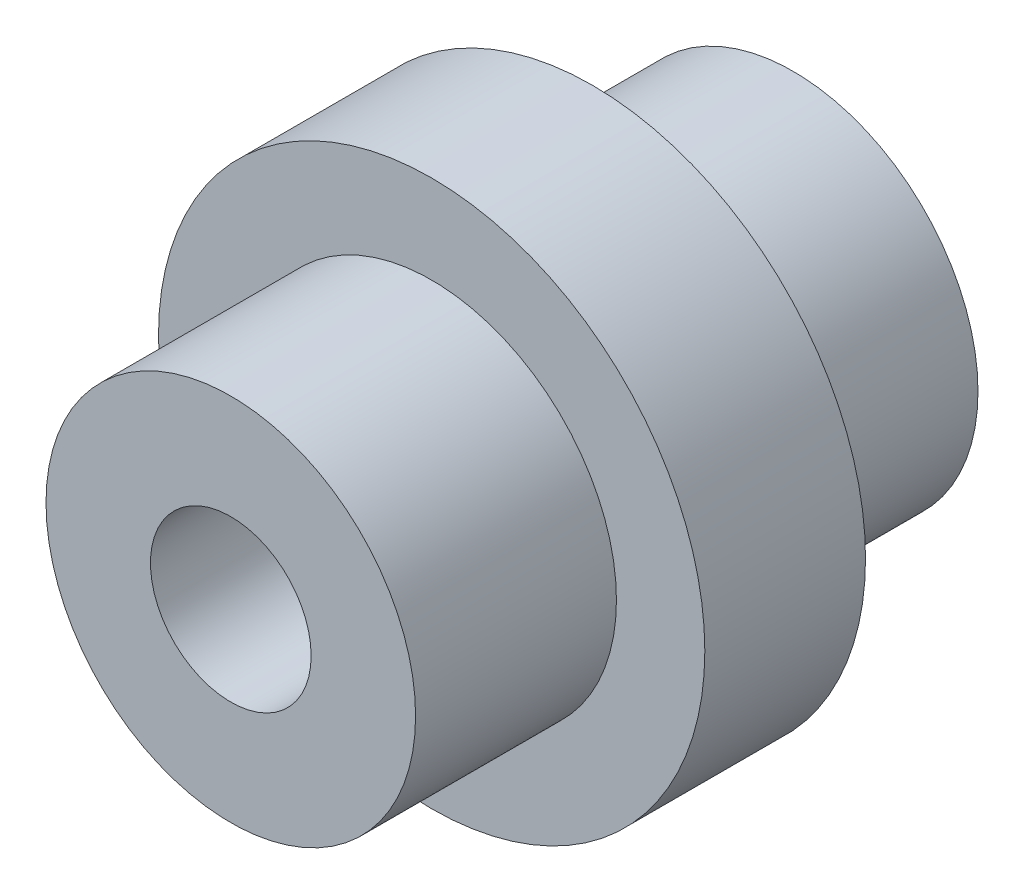
from build123d import *

# Parameters (mm, degrees)
SKETCH1_R           = 34
BOSS_EXTRUDE1_DEPTH = 10
SKETCH2_R           = 23
BOSS_EXTRUDE2_DEPTH = 25
SKETCH3_R           = 10
CUT_EXTRUDE1_DEPTH  = 17
SKETCH4_R           = 16
CUT_EXTRUDE2_DEPTH  = 17


with BuildPart() as part:
    # Sketch1 → Boss-Extrude1 (new, symmetric)
    with BuildSketch(Plane.XY):
        Circle(SKETCH1_R)
    extrude(amount=BOSS_EXTRUDE1_DEPTH, both=True)

    # Sketch2 → Boss-Extrude2 (add)
    with BuildSketch(Plane.XY.offset(10)):
        Circle(SKETCH2_R)
    boss_extrude2 = extrude(amount=BOSS_EXTRUDE2_DEPTH)

    # Mirror1: Boss-Extrude2 across plane
    add(boss_extrude2.mirror(Plane.XY))

    # Sketch3 → Cut-Extrude1 (cut)
    with BuildSketch(Plane.XY.offset(35)):
        Circle(SKETCH3_R)
    extrude(amount=-CUT_EXTRUDE1_DEPTH, mode=Mode.SUBTRACT)

    # Sketch4 → Cut-Extrude2 (cut)
    with BuildSketch(Plane(origin=(0, 0, -35), x_dir=(-1, 0, 0), z_dir=(0, 0, -1))):
        Circle(SKETCH4_R)
    extrude(amount=-CUT_EXTRUDE2_DEPTH, mode=Mode.SUBTRACT)


solid = part.part
